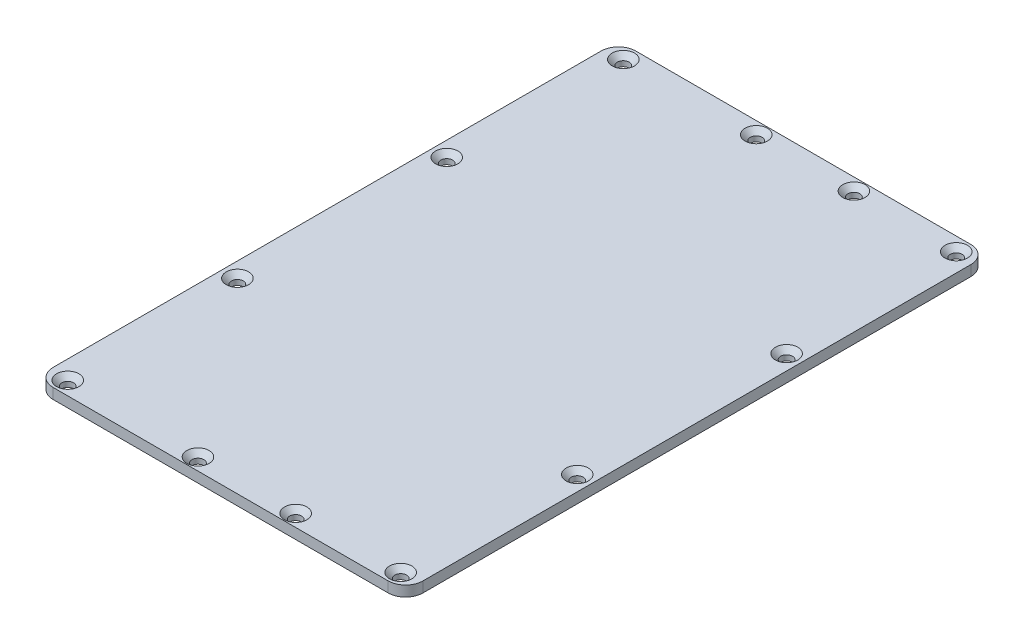
from build123d import *

# Parameters (mm, degrees)
BOSS_EXTRUDE1_DEPTH                                  = 3
HOLE_SIZE_FOR_SLOTTED_COUNTERSUNK_HEAD_S_D           = 3.4
HOLE_SIZE_FOR_SLOTTED_COUNTERSUNK_HEAD_S_DEPTH       = 13.5
HOLE_SIZE_FOR_SLOTTED_COUNTERSUNK_HEAD_S_CSINK_D     = 6.4
HOLE_SIZE_FOR_SLOTTED_COUNTERSUNK_HEAD_S_CSINK_ANGLE = 90
HOLE_SIZE_FOR_SLOTTED_COUNTERSUNK_HEAD_S_TIP         = 1.021463052


with BuildPart() as part:
    # Sketch1 → Boss-Extrude1 (new body)
    with BuildSketch(Plane(origin=(0, 0, 0), x_dir=(1, 0, 0), z_dir=(0, 1, 0))):
        with BuildLine():
            Line((84.656225745, 11.009032059), (84.656225745, 168.009032059))
            ThreePointArc((84.656225745, 168.009032059), (83.191759651, 171.544565965), (79.656225745, 173.009032059))
            Line((79.656225745, 173.009032059), (-16.343774255, 173.009032059))
            ThreePointArc((-16.343774255, 173.009032059), (-19.879308161, 171.544565965), (-21.343774255, 168.009032059))
            Line((-21.343774255, 168.009032059), (-21.343774255, 11.009032059))
            ThreePointArc((-21.343774255, 11.009032059), (-19.879308161, 7.473498153), (-16.343774255, 6.009032059))
            Line((-16.343774255, 6.009032059), (79.656225745, 6.009032059))
            ThreePointArc((79.656225745, 6.009032059), (83.191759651, 7.473498153), (84.656225745, 11.009032059))
        make_face()
    extrude(amount=BOSS_EXTRUDE1_DEPTH)

    # Hole size for slotted countersunk head screw type 0
    with Locations(Plane(origin=(0, 3, 0), x_dir=(1, 0, 0), z_dir=(0, 1, 0))):
        with Locations((-16.052531466, 169.11778927), (79.364982956, 169.11778927), (80.356225745, 119.509032059), (80.356225745, 59.509032059), (79.364982956, 9.900274848), (-16.052531466, 9.900274848), (-17.043774255, 59.509032059), (-17.043774255, 119.509032059), (21.656225745, 169.509032059), (49.656225745, 169.509032059), (21.656225745, 9.509032059), (49.656225745, 9.509032059)):
            CounterSinkHole(HOLE_SIZE_FOR_SLOTTED_COUNTERSUNK_HEAD_S_D / 2, HOLE_SIZE_FOR_SLOTTED_COUNTERSUNK_HEAD_S_CSINK_D / 2, depth=HOLE_SIZE_FOR_SLOTTED_COUNTERSUNK_HEAD_S_DEPTH, counter_sink_angle=HOLE_SIZE_FOR_SLOTTED_COUNTERSUNK_HEAD_S_CSINK_ANGLE)
            with Locations((0, 0, -(HOLE_SIZE_FOR_SLOTTED_COUNTERSUNK_HEAD_S_DEPTH + HOLE_SIZE_FOR_SLOTTED_COUNTERSUNK_HEAD_S_TIP / 2))):  # 118° drill point
                Cone(0, HOLE_SIZE_FOR_SLOTTED_COUNTERSUNK_HEAD_S_D / 2, HOLE_SIZE_FOR_SLOTTED_COUNTERSUNK_HEAD_S_TIP, mode=Mode.SUBTRACT)


solid = part.part
